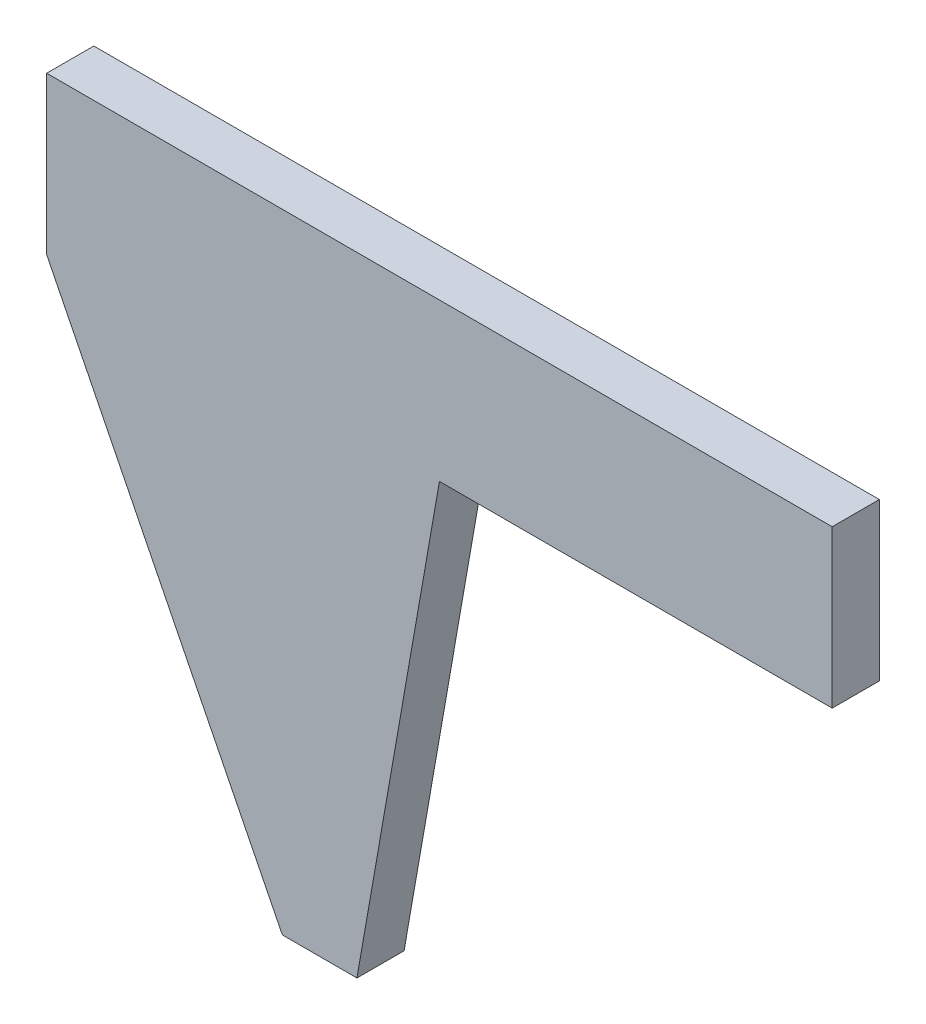
SolidWorks part; units mm, degrees
material "1023 碳钢板 (SS)"
ref_plane "前视基准面" through (0, 0, 0) normal (0, 0, 1) x (1, 0, 0)
ref_plane "上视基准面" through (0, 0, 0) normal (0, 1, 0) x (1, 0, 0)
ref_plane "右视基准面" through (0, 0, 0) normal (1, 0, 0) x (0, 0, -1)
sketch "草图1" plane through (0, 0, 0) normal (0, 0, 1) x (1, 0, 0)
  line L1 (100, 80) -> (-100, 80)
  line L2 (100, 80) -> (100, -80)
  line L3 (100, -80) -> (-100, -80)
  line L4 (-100, 80) -> (-100, -80)
  line L5 (100, 80) -> (-100, -80) construction
  line L6 (100, -80) -> (-100, 80) construction
  point P0 (0, 0)
  dimension "D1" = 200
  dimension "D2" = 160
extrude "凸台-拉伸1" add sketch "草图1" along normal blind 12
sketch "草图2" plane through (0, 0, 12) normal (0, 0, 1) x (1, 0, 0)
  line L0 (-100, 40) -> (-40, -80)
  line L1 (-100, 80) -> (-100, -80) construction
  line L2 (-100, -80) -> (100, -80) construction
  line L3 (-40, -80) -> (-100, -80)
  line L4 (-100, -80) -> (-100, 40)
  line L5 (-21, -80) -> (0, 40)
  line L6 (0, 40) -> (100, 40)
  line L7 (100, -80) -> (100, 80) construction
  line L8 (100, 40) -> (100, -80)
  line L9 (100, -80) -> (-21, -80)
  dimension "D1" = 60
  dimension "D2" = 120
  dimension "D3" = 19
  dimension "D4" = 120
  dimension "D5" = 100
extrude "切除-拉伸1" cut sketch "草图2" against normal blind 12
